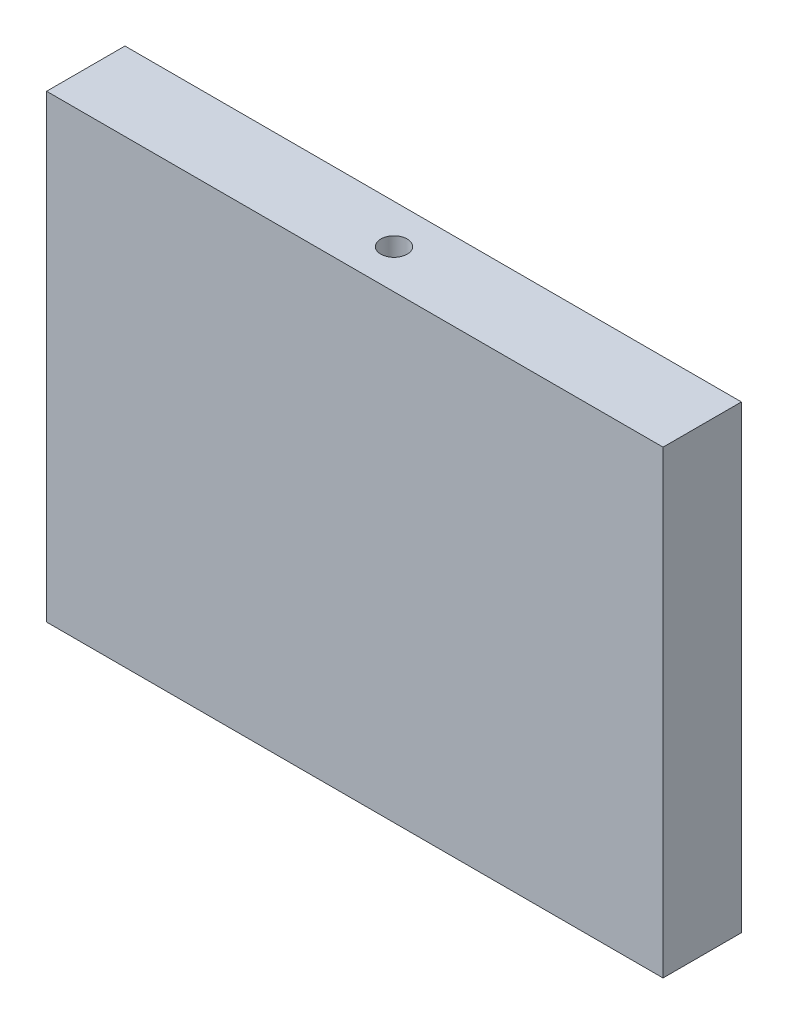
SolidWorks part; units mm, degrees
ref_plane "Front Plane" through (0, 0, 0) normal (0, 0, 1) x (1, 0, 0)
ref_plane "Top Plane" through (0, 0, 0) normal (0, 1, 0) x (1, 0, 0)
ref_plane "Right Plane" through (0, 0, 0) normal (1, 0, 0) x (0, 0, -1)
sketch "Sketch1" plane through (0, 0, 0) normal (0, 0, 1) x (1, 0, 0)
  line L1 (118, 88) -> (-118, 88)
  line L2 (118, 88) -> (118, -88)
  line L3 (118, -88) -> (-118, -88)
  line L4 (-118, 88) -> (-118, -88)
  line L5 (118, 88) -> (-118, -88) construction
  line L6 (118, -88) -> (-118, 88) construction
  point P0 (0, 0)
  dimension "D1" = 236
  dimension "D2" = 176
extrude "Boss-Extrude1" add sketch "Sketch1" along normal blind 30
sketch "Sketch3" plane through (0, 88, 0) normal (0, 1, 0) x (1, 0, 0)
  line L0 (-118, -30) -> (-118, 0) construction
  circle A0 centre (0, -15) radius 5.055
  point P4 (-118, -15)
  dimension "D1" = 10.11
extrude "Cut-Extrude1" cut sketch "Sketch3" against normal through all
